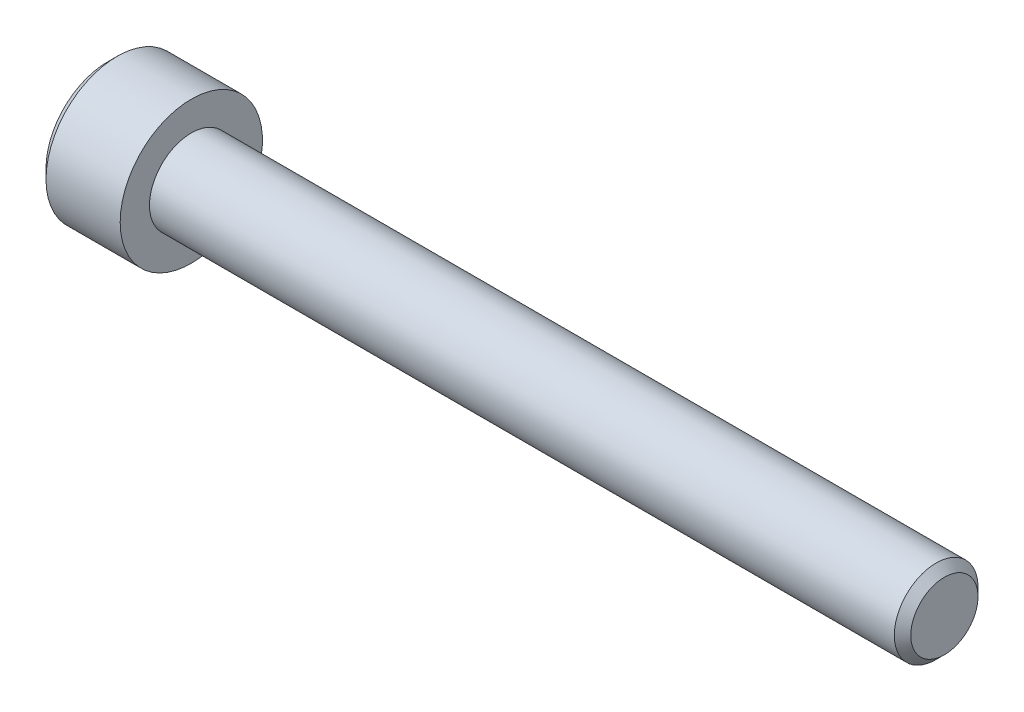
from build123d import *

# Parameters (mm, degrees)
CUT_EXTRUDE1_DEPTH = 2.5


with BuildPart() as part:
    # Sketch1 → Revolve1 (revolve)
    with BuildSketch(Plane.XY, mode=Mode.PRIVATE) as revolve1_sk:
        Polygon((-5, 0), (-5, 3.683333333), (-4.433333333, 4.25), (0, 4.25), (0, 2.5), (44.508532, 2.5), (45, 2.008532), (45, 0), align=None)
    revolve(revolve1_sk.sketch.rotate(Axis((45, 0, 0), (-1, 0, 0)), 270), axis=Axis((45, 0, 0), (-1, 0, 0)))

    # Sketch2 → Cut-Revolve1 (revolve, cut)
    with BuildSketch(Plane.XY, mode=Mode.PRIVATE) as cut_revolve1_sk:
        Polygon((-5, 0), (-5, 2), (-2.5, 2), (-1.964101615, 0), align=None)
    revolve(cut_revolve1_sk.sketch.rotate(Axis((-1.964101615, 0, 0), (-1, 0, 0)), 270), axis=Axis((-1.964101615, 0, 0), (-1, 0, 0)), mode=Mode.SUBTRACT)

    # Sketch3 → Cut-Extrude1 (cut)
    with BuildSketch(Plane(origin=(-5, 0, 0), x_dir=(0, 0, -1), z_dir=(1, 0, 0))):
        Polygon((-2, 1.154700538), (-2, -1.154700538), (0, -2.309401077), (2, -1.154700538), (2, 1.154700538), (0, 2.309401077), align=None)
    extrude(amount=CUT_EXTRUDE1_DEPTH, mode=Mode.SUBTRACT)


solid = part.part
